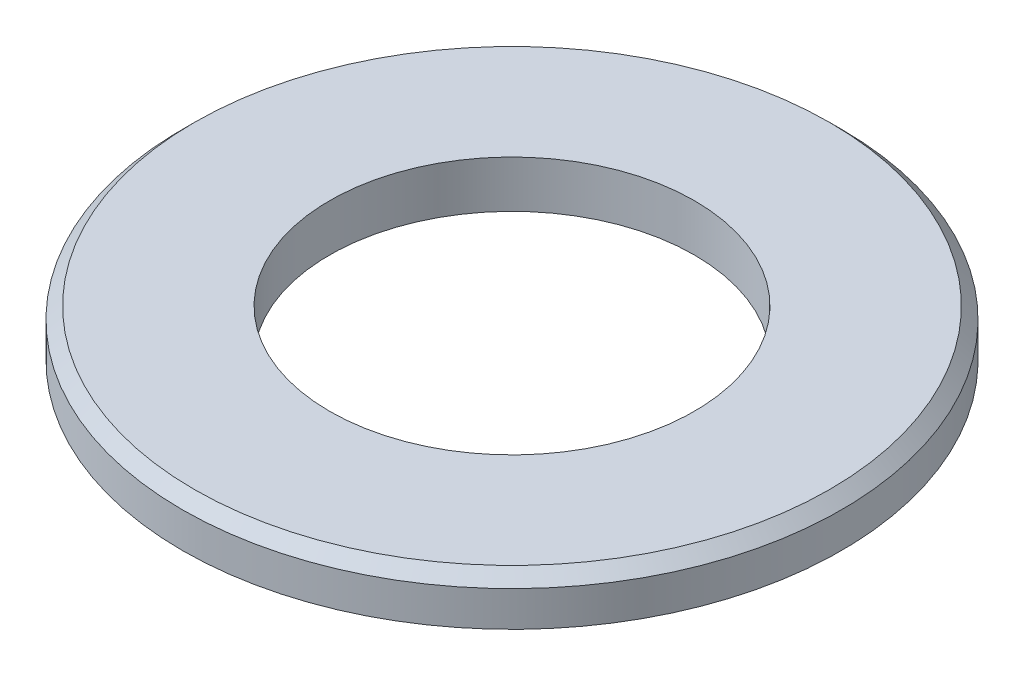
from build123d import *


with BuildPart() as part:
    # 草图1 → Revolve 432 (revolve)
    with BuildSketch(Plane.XY, mode=Mode.PRIVATE) as revolve_432_sk:
        Polygon((-27, 12.644507042), (-28, 11.644507042), (-28, 8.644507042), (-15.5, 8.644507042), (-15.5, 12.644507042), align=None)
    revolve(revolve_432_sk.sketch.rotate(Axis((0, 0, 0), (0, 1, 0)), 270), axis=Axis((0, 0, 0), (0, 1, 0)))


solid = part.part
